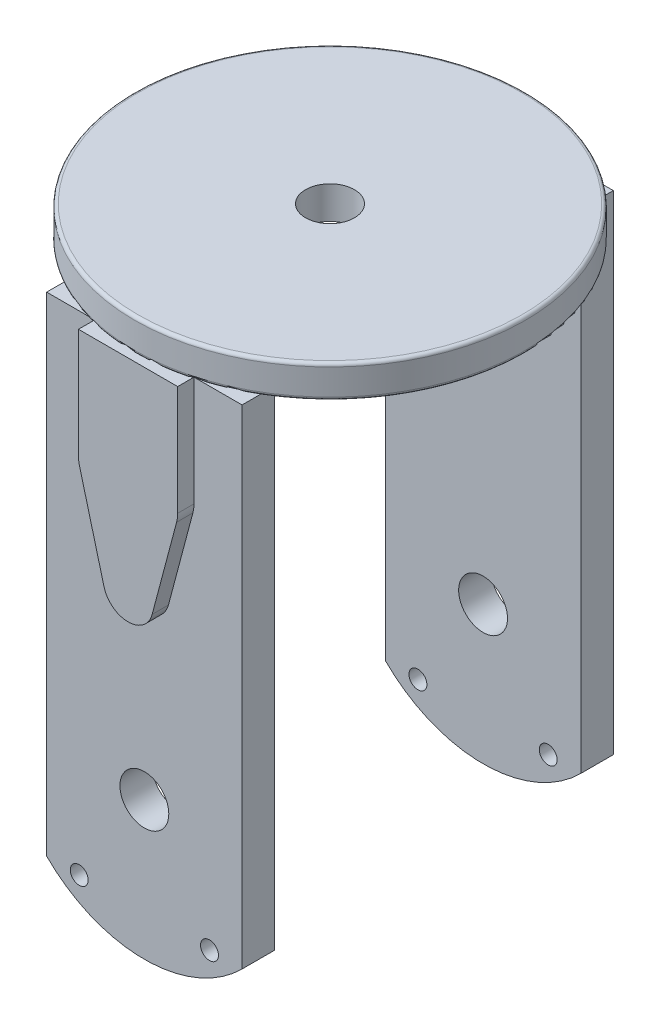
SolidWorks part; units mm, degrees
ref_plane "Front Plane" through (0, 0, 0) normal (0, 0, 1) x (1, 0, 0)
ref_plane "Top Plane" through (0, 0, 0) normal (0, 1, 0) x (1, 0, 0)
ref_plane "Right Plane" through (0, 0, 0) normal (1, 0, 0) x (0, 0, -1)
sketch "Sketch1" plane through (0, 0, 0) normal (0, 1, 0) x (1, 0, 0)
  line L0 (0, 60) -> (0, -60) construction
  line L1 (-60, 0) -> (60, 0) construction
  circle A0 centre (0, 0) radius 60
  dimension "D1" = 120
extrude "Boss-Extrude1" add sketch "Sketch1" along normal blind 10
fillet "Fillet2" radius 1 2 edges at (0, 0, 60) (0, 10, 60)
ref_plane "Plane1" through (0, 0, 47) normal (0, 0, 1) x (1, 0, 0)
sketch "Sketch2" plane through (0, 0, 47) normal (0, 0, 1) x (1, 0, 0)
  line L1 (-59, 0) -> (59, 0) construction
  line L3 (0, 0) -> (0, -165.1329) construction
  line L7 (30, 0) -> (-30, 0)
  line L9 (-30, -150) -> (-30, 0)
  line L14 (30, -150) -> (-30, -150) construction
  line L15 (30, -150) -> (30, 0)
  arc A9 (-30, -150) -> (30, -150) centre (0, -120) ccw
  circle A10 centre (0, -120) radius 7.5
  dimension "D3" = 120
  dimension "D4" = 15
  dimension "D1" = 30
  dimension "D2" = 150
sketch "Sketch5" plane through (0, 10, 0) normal (0, 1, 0) x (1, 0, 0)
  circle A0 centre (0, 0) radius 7.5
  dimension "D1" = 15
extrude "Cut-Extrude2" cut sketch "Sketch5" against normal through all
extrude "Boss-Extrude2" add sketch "Sketch2" along normal blind 10
sketch "Sketch7" plane through (0, 0, 57) normal (0, 0, 1) x (1, 0, 0)
  line L0 (-15.2315, 0) -> (15.2315, 0)
  line L1 (15.2315, 0) -> (15.2315, -33.6945)
  line L2 (14.8964, -36.2617) -> (7.3939, -64.5062)
  line L3 (-15.2315, 0) -> (-15.2315, -33.6945)
  line L6 (-14.8964, -36.2617) -> (-7.3939, -64.5062)
  arc A0 (-7.3939, -64.5062) -> (7.3939, -64.5062) centre (0, -62.5421) ccw
  arc A1 (-14.8964, -36.2617) -> (-15.2315, -33.6945) centre (-5.2315, -33.6945) cw
  arc A3 (14.8964, -36.2617) -> (15.2315, -33.6945) centre (5.2315, -33.6945) ccw
  point P13 (-15.2315, -35)
  dimension "D1" = 10
  dimension "D2" = 10
extrude "Boss-Extrude4" add sketch "Sketch7" along normal blind 5
ref_plane "Plane2" through (0, 0, -60) normal (0, 0, -1) x (-1, 0, 0)
ref_plane "Plane3" through (0, 0, 60) normal (0, 0, 1) x (1, 0, 0)
ref_plane "Plane4" through (0, 0, 0) normal (0, 0, 1) x (1, 0, 0)
mirror "Mirror2" about plane through (0, 0, 0) normal (0, 0, 1) of "Cut-Extrude2", "Boss-Extrude2", "Boss-Extrude4"
sketch "Sketch9" plane through (0, 0, -60) normal (0, 0, -1) x (-1, 0, 0)
  line L0 (-30, -150) -> (30, -150) construction
  line L1 (30, 0) -> (30, -150) construction
  line L2 (0, -120) -> (0, -162.4264) construction
  arc A0 (-30, -150) -> (30, -150) centre (0, -120) ccw construction
  point P12 (-20, -150)
  dimension "D1" = 10
hole_wizard "CBORE for M5 Hexagon head bolts-Full thread-grade C1" positions "Sketch9" profile "Sketch10" counterbore size "M5" standard "GB" end condition through all
sketch "Sketch10" plane through (20, -150, -60) normal (1, 0, 0) x (0, 1, 0)
  line L0 (0, 0) -> (0, 122)
  line L1 (0, 122) -> (2.75, 122)
  line L3 (2.75, 122) -> (2.75, 0.5)
  line L4 (5.5, 0.5) -> (2.75, 0.5)
  line L5 (5.5, 0.5) -> (5.5, 0.025)
  line L6 (5.5, 0.025) -> (5.525, 0)
  line L7 (5.525, 0) -> (0, 0)
  line L8 (-5.5, 0.025) -> (-5.525, 0) construction
  line L11 (0, -6.35) -> (0, 107.95) construction
  dimension "通孔孔直径" = 5.5
  dimension "通孔孔深度" = 122
  dimension "柱形沉头孔直径" = 11
  dimension "柱形沉头孔深度" = 0.5
  dimension "近端锥形沉头孔直径" = 11.05
  dimension "近端锥形沉头孔角度" = 90
ref_plane "Plane5" through (0, 0, 0) normal (-1, 0, 0) x (0, 0, 1)
mirror "Mirror3" about plane through (0, 0, 0) normal (-1, 0, 0) of "CBORE for M5 Hexagon head bolts-Full thread-grade C1"
